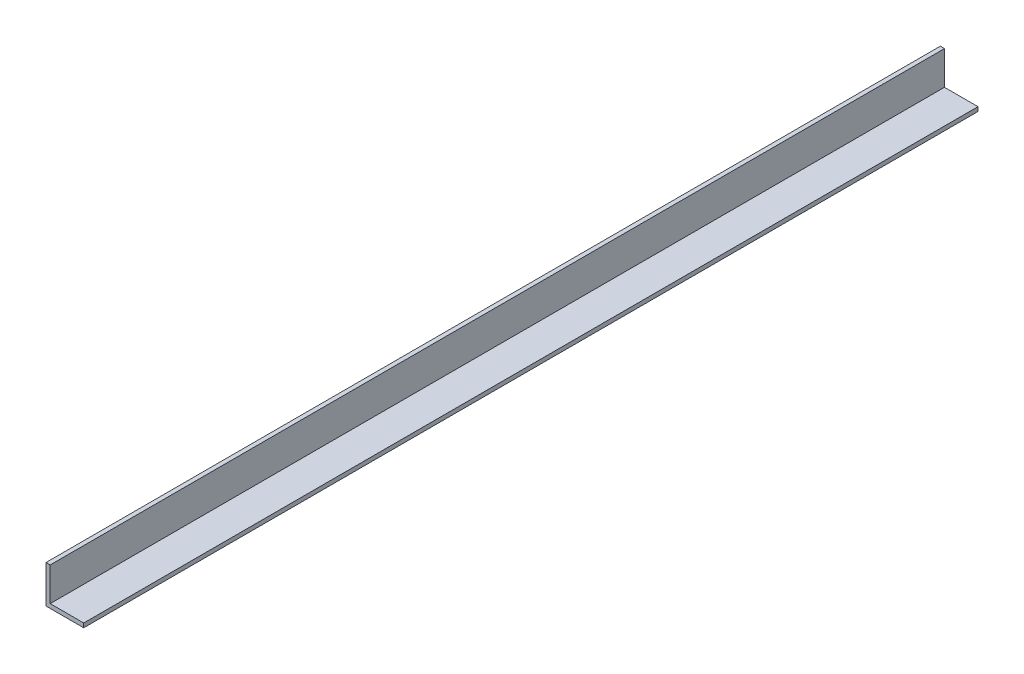
SolidWorks part; units mm, degrees
material "1023 碳钢板 (SS)"
ref_plane "Front Plane" through (0, 0, 0) normal (0, 0, 1) x (1, 0, 0)
ref_plane "Top Plane" through (0, 0, 0) normal (0, 1, 0) x (1, 0, 0)
ref_plane "Right Plane" through (0, 0, 0) normal (1, 0, 0) x (0, 0, -1)
sketch "Sketch1" plane through (0, 0, 0) normal (0, 0, 1) x (1, 0, 0)
  line L0 (-24.6495, 21.9527) -> (-24.6495, -23.0473)
  line L1 (-24.6495, -23.0473) -> (20.3505, -23.0473)
  line L2 (20.3505, -23.0473) -> (20.3505, -18.0473)
  line L3 (20.3505, -18.0473) -> (-19.6495, -18.0473)
  line L4 (-19.6495, -18.0473) -> (-19.6495, 21.9527)
  line L5 (-19.6495, 21.9527) -> (-24.6495, 21.9527)
  dimension "D1" = 5
  dimension "D2" = 5
  dimension "D3" = 45
  dimension "D4" = 45
extrude "Extrude1" add sketch "Sketch1" along normal blind 1066.8
